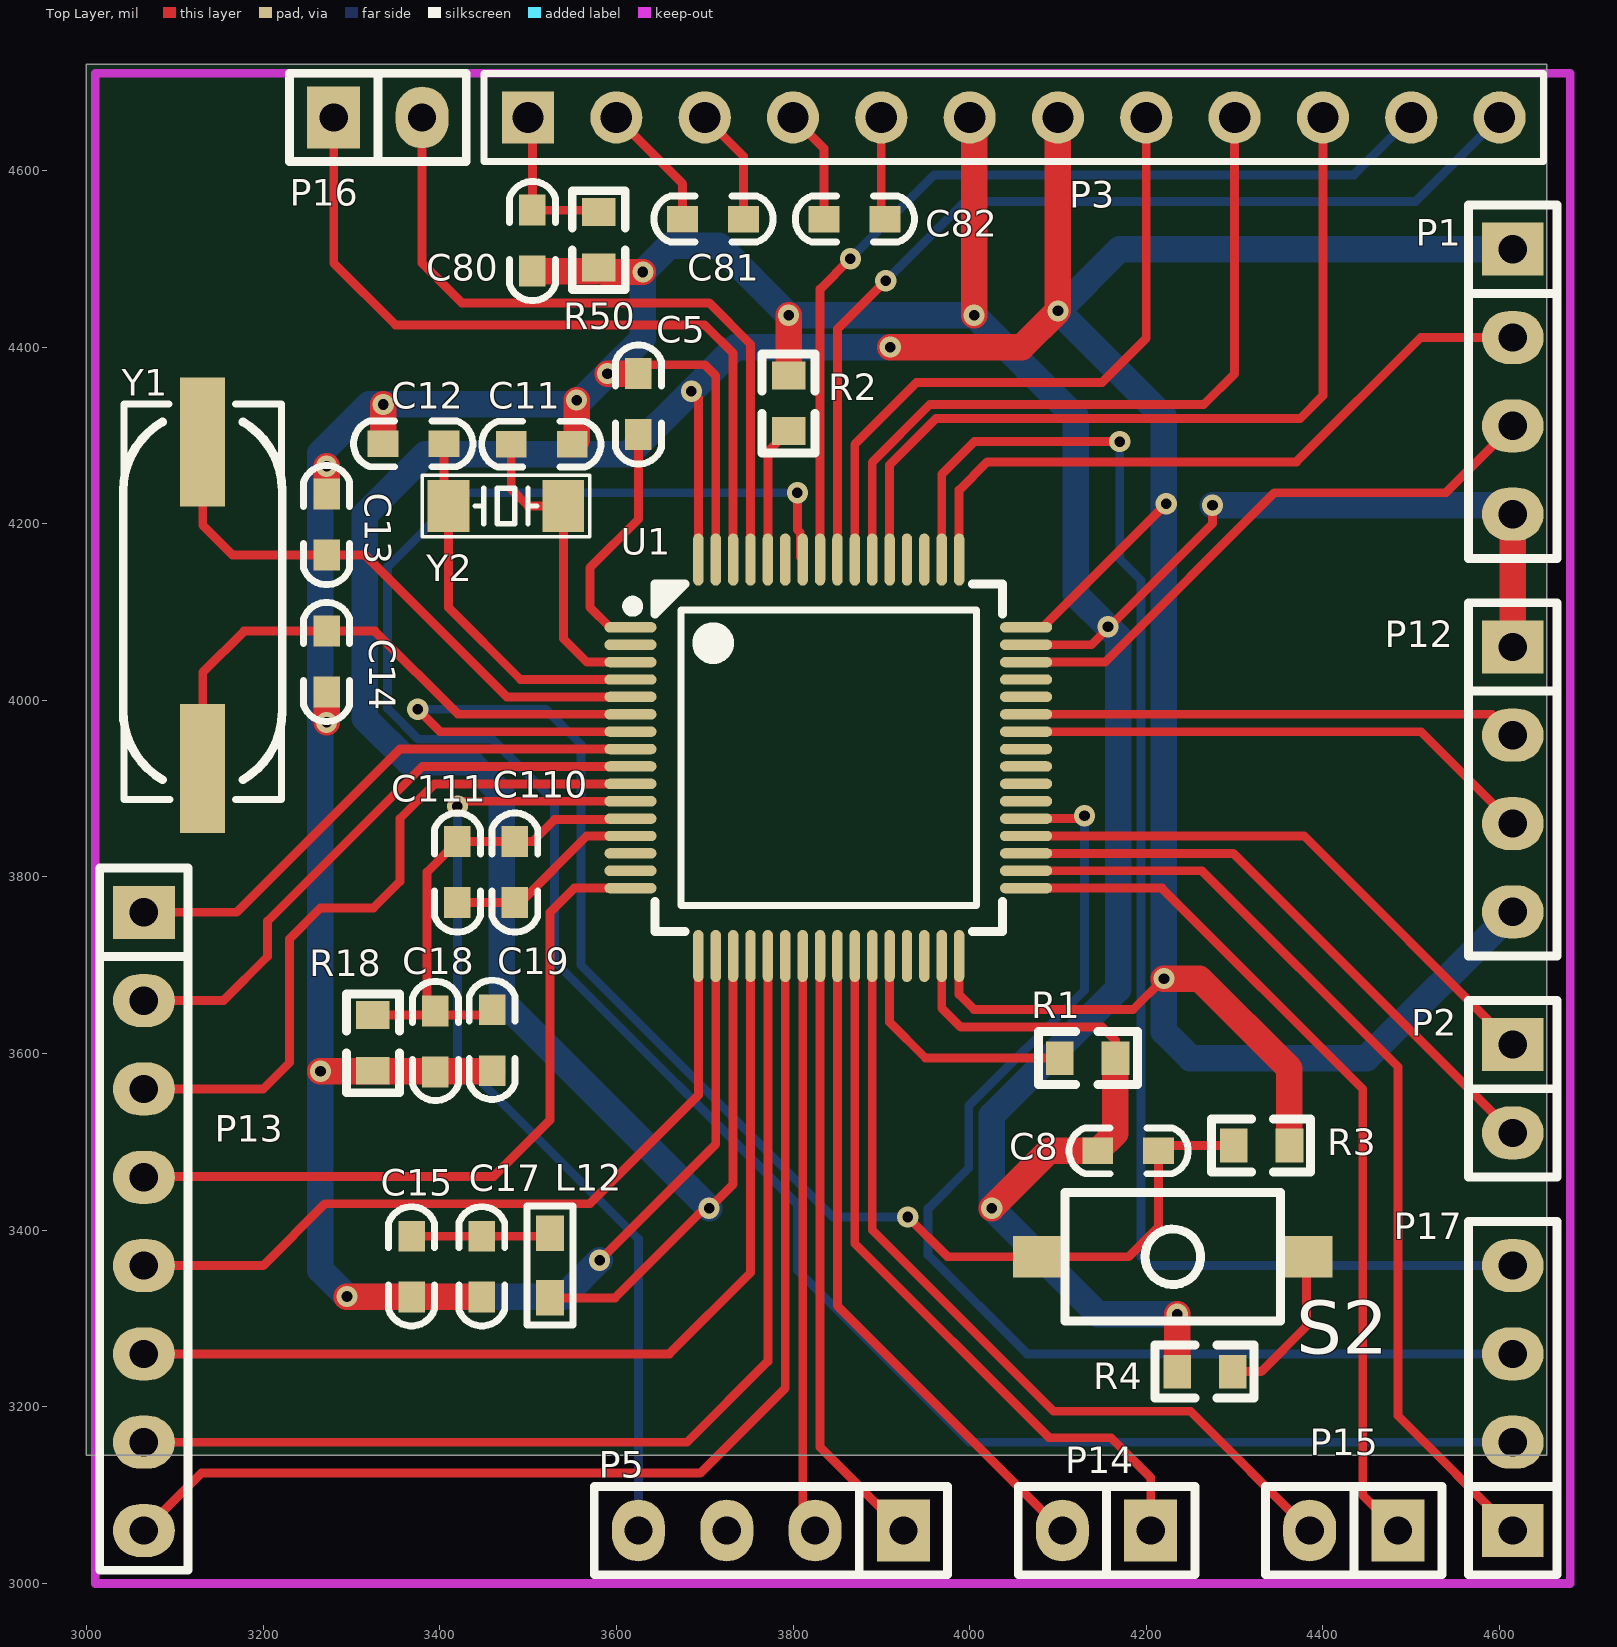
[diagram p0: Top Layer view]
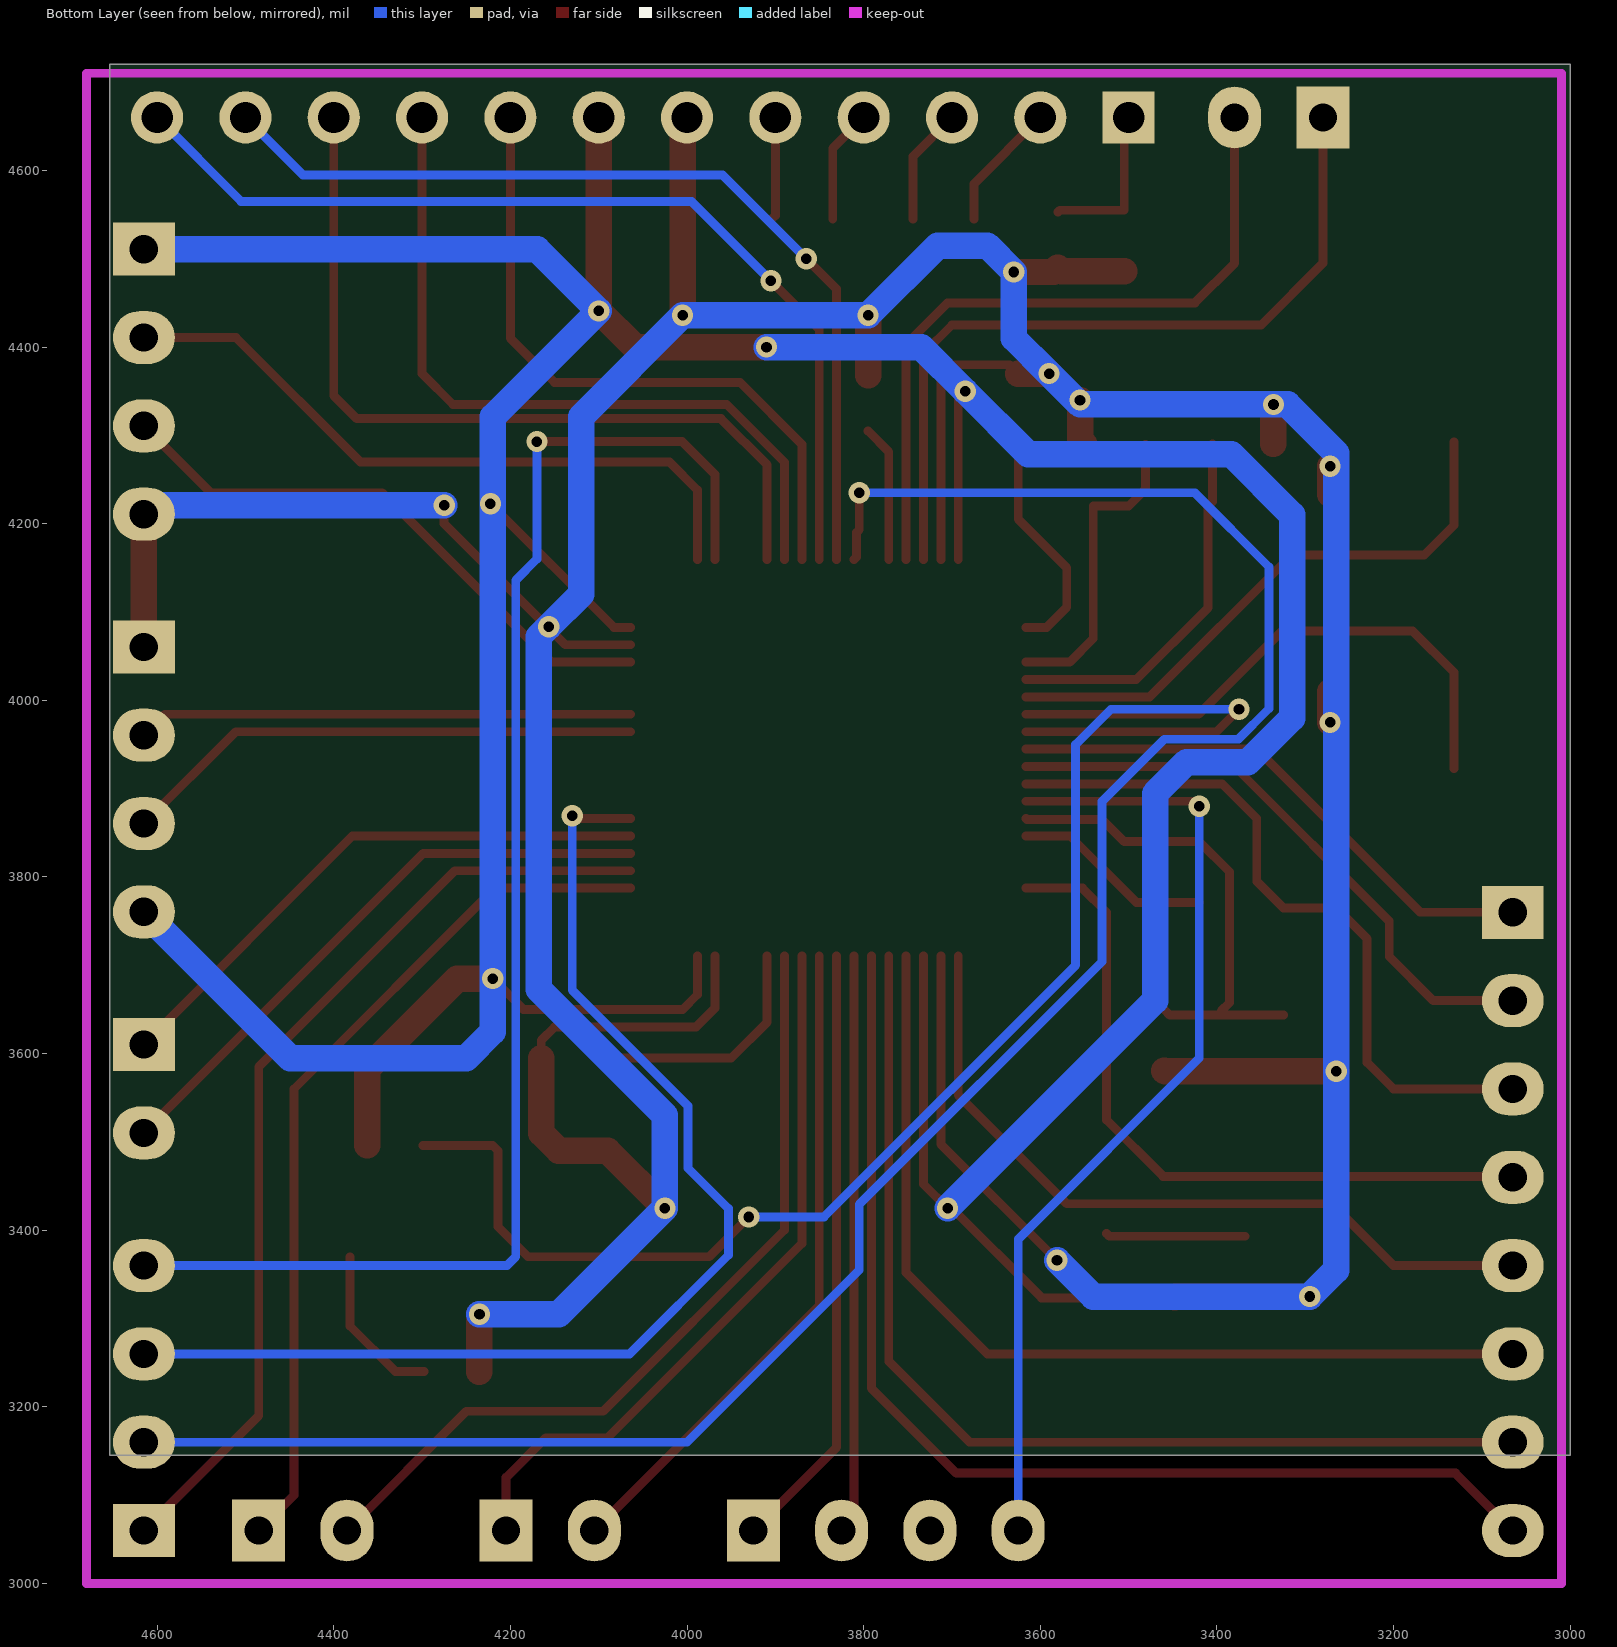
[diagram p1: Bottom Layer view, seen from below]
# Altium PCB MISC51920.pcbdoc
Units mil, origin at the board's own origin, x right, y up, seen from the top; angles counter-clockwise.
Board outline 1653.54 x 1574.8 mil, 2 copper layers (Top Layer, Bottom Layer); 36 components, 70 nets, 158 pads, 29 vias.

## Layer stack, top to bottom (the 12.6 mil dielectric is the usual default, probably not edited)
Top Solder Mask Layer: solder mask 1.4, FR-4, Dk 4.8
Top Layer: signal copper 1.4
Substrate1: surface 12.6, FR-4, Dk 4.8
Bottom Layer: signal copper 1.4
Bottom Solder Mask Layer: solder mask 1.4, FR-4, Dk 4.8

## Board outline
4653.54,3145.2 3000,3145.2 3000,4720 4653.54,4720

## Design rules (kind name [scope] priority, off if disabled: settings)
BoardOutlineClearance Clearance_1 [All] p2: genericclearance=6 ignorepadtopadclearanceinfootprint=FALSE except(0: Arc-SplitContinuation Track-SplitContinuation SMDPad-SplitContinuation THPad-SplitContinuation Via-SplitContinuation Fill-SplitContinuation Region-SplitContinuation Poly-SplitContinuation Text-SplitContinuation Hole-SplitContinuation; 6: Arc-OutlineEdge Track-OutlineEdge SMDPad-OutlineEdge THPad-OutlineEdge Via-OutlineEdge Fill-OutlineEdge Region-OutlineEdge Poly-OutlineEdge Text-OutlineEdge Hole-OutlineEdge SMDPad-CutoutEdge THPad-CutoutEdge Via-CutoutEdge Fill-CutoutEdge Region-CutoutEdge Poly-CutoutEdge Text-CutoutEdge; 6.9: Hole-CutoutEdge; 11.8: Arc-CutoutEdge Track-CutoutEdge)
Clearance [All] p1: gap=6 ignorepadtopadclearanceinfootprint=FALSE
Creepage creepage [All] p1: checkdistance=0 ignoreinternallayers=TRUE applytopolygonpour=TRUE
DiffPairsRouting [All] p1: maxlimit=10 minlimit=6 mostfreqgap=6 toplayer_minwidth=0 toplayer_prefwidth=0 toplayer_maxwidth=0 toplayer_mingap=10 toplayer_prefgap=10 toplayer_maxgap=10 bottomlayer_minwidth=0 bottomlayer_prefwidth=0 bottomlayer_maxwidth=0 bottomlayer_mingap=10 bottomlayer_prefgap=10 bottomlayer_maxgap=10 maxuncoupledlength=10
HoleToHoleClearance ComponentClearance [All] p1: gap=11.81 allowstackedmicrovias=TRUE
Length netLength [All] p1: minlimit=0 maxlimit=0
MatchedLengths netLengthTolerance [All] p1: tolerance=1000
PolygonConnect [(InNet('TIM3_CH1') OR InNet('ADC_IN14'))] p1: connectstyle=Relief reliefconductorwidth=10 reliefentries=4 polygonreliefangle="90 Angle" airgapwidth=10 via.connectstyle=Relief via.reliefconductorwidth=10 via.reliefentries=4 via.polygonreliefangle="90 Angle" via.airgapwidth=10
RoutingVias [All] p1: holewidth=15 width=30 viastyle="Through Hole" minholewidth=12 minwidth=22 maxholewidth=15 maxwidth=30
SolderMaskExpansion [All] p1: expansion=4 istentingtop=FALSE
Width [All] p1: maxlimit=10 minlimit=10 preferedwidth=10 toplayer_minwidth=8 toplayer_maxwidth=30 toplayer_prefwidth=10 bottomlayer_minwidth=8 bottomlayer_maxwidth=30 bottomlayer_prefwidth=10
2 further rules are at their usual default settings.

## Components (designator, comment, footprint, x,y, rotation, side; value= is the part's Value field where it differs from the comment)
C5 "1uF" "C 0603" 3625,4335 r270 top
C8 "104" "C 0603" 4180,3490 r0 top
C11 "20P" "C 0603" 3515,4290 r180 top
C12 "20P" "C 0603" 3370,4290.51 r180 top
C13 "20P" "C 0603" 3271.92,4198.46 r270 top
C14 "20P" "C 0603" 3271.92,4043.46 r270 top
C15 "1uF" "C 0603" 3368.05,3359.22 r90 top
C17 "0.01uF" "C 0603" 3447.61,3359.22 r90 top
C18 "1uF" "C 0603" 3395.19,3614.41 r90 top
C19 "0.01uF" "C 0603" 3459.41,3615.66 r90 top
C80 "330pF" "C 0603" 3505,4520 r270 top
C81 "2.2uF" "C 0603" 3710,4545 r0 top
C82 "2.2uF" "C 0603" 3870,4545 r0 top
C110 "0.1uF" "C 0603" 3485,3805 r270 top
C111 "0.01uF" "C 0603" 3420,3805 r270 top
L12 "2uH" "R 0603" 3525,3360 r270 top
P1 "Pin HDR1X4" "Pin HDR1X4/2.54mm-S" 4615,4510.8 r0 top
P2 "Pin HDR1X2" "Pin HDR1X2/2.54mm-S" 4615,3610.27 r0 top
P3 "Pin HDR1X12" "Pin HDR1X12/2.54mm-S" 3500,4660 r0 top
P5 "Pin HDR1X4" "Pin HDR1X4/2.54mm-S" 3925,3060 r270 top
P12 "Pin HDR1X4" "Pin HDR1X4/2.54mm-S" 4615,4060.53 r0 top
P13 "Pin HDR1X8" "Pin HDR1X8/2.54mm-S" 3065,3760 r0 top
P14 "Pin HDR1X2" "Pin HDR1X2/2.54mm-S" 4205,3060 r270 top
P15 "Pin HDR1X2" "Pin HDR1X2/2.54mm-S" 4485,3060 r270 top
P16 "Pin HDR1X2" "Pin HDR1X2/2.54mm-S" 3280,4660 r90 top
P17 "Pin HDR1X4" "Pin HDR1X4/2.54mm-S" 4615,3060 r180 top
R1 "10K" 0603R 4165,3595 r180 top
R2 "10K" 0603R 3795,4305 r90 top
R3 "10K" 0603R 4299,3496 r0 top
R4 "330R" 0603R 4235,3240 r0 top
R18 "0R" 0603R 3324.41,3580.66 r90 top
R50 "3.3-10M" 0603R 3580,4490 r90 top
S2 "KEY" SWTP3.7X6 4230,3370 r180 top
U1 "STM32L152RBT6" LQFP-64_L10.0-W10.0-P0.50-LS12.0-BL 3840,3935 r270 top
Y1 "8MHz" XTAL_SMD49S 3131.6,3922.69 r270 top
Y2 "32.768kHz" "OSC 3215-2P" 3475,4220 r180 top

## Footprints (in the part's own frame and the unit in brackets; to place one, negate y for a bottom-side part, rotate by r counter-clockwise, add the part's x,y. Pads: shape width x height; smd on the part's side, far side on the other; paste and mask are expansions set on the pad)
0603R [mm]
  rect 0.8x0.965 smd: 1(0,0) 2(1.6,0)
  silkscreen extent -0.64,-0.76 2.21,0.76
"C 0603" [mil]
  rect 35x30 smd: 1(-35,0) 2(34,0)
  silkscreen extent -67,-26 67,26
LQFP-64_L10.0-W10.0-P0.50-LS12.0-BL [mm]
  oval 0.3x1.5 smd: 1(-3.75,-5.688) 2(-3.25,-5.688) 3(-2.75,-5.688) 4(-2.25,-5.688) 5(-1.75,-5.688) 6(-1.25,-5.688) 7(-0.75,-5.688) 8(-0.25,-5.688) 9(0.25,-5.688) 10(0.75,-5.688) 11(1.25,-5.688) 12(1.75,-5.688) 13(2.25,-5.688) 14(2.75,-5.688) 15(3.25,-5.688) 16(3.75,-5.688) 33(3.75,5.688) 34(3.25,5.688) 35(2.75,5.688) 36(2.25,5.688) 37(1.75,5.688) 38(1.25,5.688) 39(0.75,5.688) 40(0.25,5.688) 41(-0.25,5.688) 42(-0.75,5.688) 43(-1.25,5.688) 44(-1.75,5.688) 45(-2.25,5.688) 46(-2.75,5.688) 47(-3.25,5.688) 48(-3.75,5.688)
  oval 1.5x0.3 smd: 17(5.7,-3.738) 18(5.7,-3.238) 19(5.7,-2.738) 20(5.7,-2.238) 21(5.7,-1.738) 22(5.7,-1.238) 23(5.7,-0.738) 24(5.7,-0.238) 25(5.7,0.262) 26(5.7,0.762) 27(5.7,1.262) 28(5.7,1.762) 29(5.7,2.262) 30(5.7,2.762) 31(5.7,3.262) 32(5.7,3.762) 49(-5.7,3.762) 50(-5.7,3.262) 51(-5.7,2.762) 52(-5.7,2.262) 53(-5.7,1.762) 54(-5.7,1.262) 55(-5.7,0.762) 56(-5.7,0.262) 57(-5.7,-0.238) 58(-5.7,-0.738) 59(-5.7,-1.238) 60(-5.7,-1.738) 61(-5.7,-2.238) 62(-5.7,-2.738) 63(-5.7,-3.238) 64(-5.7,-3.738)
  silkscreen extent -5,-5.78 5,5.01
"OSC 3215-2P" [mm]
  rect 1.2x1.5 smd: 1(-1.65,0) 2(1.65,0)
  silkscreen extent -2.41,-0.89 2.41,0.89
"Pin HDR1X2/2.54mm-S" [mil]
  rect 70x60 hole 32: 1(0,0)
  oval 70x60 hole 32: 2(0,-100)
  silkscreen extent -50,-150 50,50
"Pin HDR1X4/2.54mm-S" [mil]
  rect 70x60 hole 32: 1(0,0)
  oval 70x60 hole 32: 2(0,-100) 3(0,-200) 4(0,-300)
  silkscreen extent -50,-350 50,50
"Pin HDR1X8/2.54mm-S" [mil]
  rect 70x60 hole 32: 1(0,0)
  oval 70x60 hole 32: 2(0,-100) 3(0,-200) 4(0,-300) 5(0,-400) 6(0,-500) 7(0,-600) 8(0,-700)
  silkscreen extent -50,-745 50,50
"Pin HDR1X12/2.54mm-S" [mm]
  rect 1.5x1.5 hole 0.9: 1(0,0)
  round 1.5 hole 0.9: 2(2.54,0) 3(5.08,0) 4(7.62,0) 5(10.16,0) 6(12.7,0) 7(15.24,0) 8(17.78,0) 9(20.32,0) 10(22.86,0) 11(25.4,0) 12(27.94,0)
  silkscreen extent -1.27,-1.27 29.21,1.27
"R 0603" [mil]
  rect 40x31.5 smd: 1(-36.5,0) 2(36.5,0)
  silkscreen extent -68,-26 68,26
SWTP3.7X6 [mm]
  rect 1.5x1.2 smd: 1(-3.85,0) 2(3.85,0)
  silkscreen extent -3.1,-1.85 3.1,1.85
XTAL_SMD49S [mil]
  rect 146x51 smd: 1(0,0) 2(-370,0)
  silkscreen extent -413,-90 35,90

## Via types
v1: diameter 24.02, hole 12, Top Layer to Bottom Layer, 29 vias

## Nets (pads, with @x,y where several pads share a name; then routed paths per layer and width w, separated by ;. In a path a pad name is that pad's centre, name@x,y a point inside that pad or via, vN(x,y) a via of type N, cw(c..) or ccw(c..) an arc to the next point about the centre after c; other vN are vias at no path point)
+3.3V: L12.2 P1.1 P3.7 P12.4 R3.2 U1.19 U1.32 U1.48 U1.64 | length 5468.9
  Top Layer w10: L12.2 3598.5,3323.5 v1@3702.5,3427.5 ; v1(3685,4350) 3692.83,4342.17 U1.64 ; v1(3705,3425) 3732.2,3452.2 U1.19 ; U1.32 3988.11,3666.89 4005,3650 4185,3650 v1(4220,3685) ; U1.48 4082.64,4082.64 v1(4222.64,4222.64)
  Top Layer w30: v1(3910,4400) 4059,4400 v1(4100,4441) P3.7 ; v1(4220,3685) 4260,3685 4361.99,3583.01 R3.2
  Bottom Layer w30: v1(3705,3425) 3470,3660 3470,3894.46 3434.46,3930 3365,3930 3315,3980 3315,4210 3383.86,4278.86 3613.86,4278.86 v1(3685,4350) 3735,4400 v1(3910,4400) ; P12.4 4449.47,3595 4249.89,3595 4220,3624.89 v1(4220,3685) 4220,4321 v1(4100,4441) 4169.8,4510.8 P1.1
ADC_IN1: U1.15
ADC_IN2: P13.4 U1.16 | length 824.3
  Top Layer w10: P13.4 3065.95,3460.95 3460.95,3460.95 3525,3525 3525,3760 3552.36,3787.36 U1.16
ADC_IN3: P13.5 U1.17 | length 865.5
  Top Layer w10: P13.5 3200,3360 3270,3430 3570,3430 3692.83,3552.83 U1.17
ADC_IN4: P13.6 U1.20 | length 1083.7
  Top Layer w10: P13.6 3660,3260 3751.89,3351.89 U1.20
ADC_IN5: P13.7 U1.21 | length 1203.5
  Top Layer w10: P13.7 3680,3160 3771.57,3251.57 U1.21
ADC_IN6: P13.8 U1.22 | length 1282.4
  Top Layer w10: P13.8 3130,3125 3695,3125 3791.26,3221.26 U1.22
ADC_IN7: P5.2 U1.23 | length 656.4
  Top Layer w10: U1.23 3810.94,3074.06 P5.2
ADC_IN8: P14.1 U1.26 | length 830.4
  Top Layer w10: U1.26 3870,3385 4090,3165 4160,3165 4205,3120 P14.1
ADC_IN9: P15.2 U1.27 | length 946.6
  Top Layer w10: U1.27 3889.68,3400.32 4095,3195 4250,3195 P15.2
ADC_IN10: P13.1 U1.8 | length 627.6
  Top Layer w10: P13.1 3170,3760 3354.84,3944.84 U1.8
ADC_IN11: P13.2 U1.9 | length 684.3
  Top Layer w10: P13.2 3155,3660 3205,3710 3205,3750 3380.16,3925.16 U1.9
ADC_IN12: P13.3 U1.10 | length 817.9
  Top Layer w10: P13.3 3200,3560 3230,3590 3230,3730 3265,3765 3325,3765 3355,3795 3355,3866.21 3394.26,3905.47 U1.10
ADC_IN13: P5.4 U1.11 | length 1103.4
  Top Layer w10: v1(3420,3880) 3425.79,3885.79 U1.11
  Bottom Layer w10: v1(3420,3880) 3420,3595 3625,3390 P5.4
ADC_IN14: P5.1 U1.24 | length 689.7
  Top Layer w10: U1.24 3830.63,3154.37 P5.1
ADC_IN15: P14.2 U1.25 | length 756.1
  Top Layer w10: U1.25 3850.31,3314.69 P14.2
ADC_IN18: P15.1 U1.33 | length 991.8
  Top Layer w10: U1.33 4217.64,3787.36 4445,3560 4445,3100 P15.1
ADC_IN19: P5.3
ADC_IN20: P2.2 U1.35 | length 682.1
  Top Layer w10: U1.35 4298.54,3826.73 P2.2
ADC_IN21: P2.1 U1.36 | length 648.9
  Top Layer w10: U1.36 4378.85,3846.42 P2.1
LCD_CD: P3.10 U1.53 | length 945.4
  Top Layer w10: U1.53 3909.37,4266.74 3961.63,4319 4374,4319 4400,4345 P3.10
LCD_CS: P3.12 U1.56 | length 1109.9
  Top Layer w10: U1.56 3850.31,4420.31 v1(3905,4475)
  Bottom Layer w10: v1(3905,4475) 3995,4565 4505,4565 P3.12
LCD_D6: P3.9 U1.54 | length 852.1
  Top Layer w10: U1.54 3889.68,4269.68 3955,4335 4265,4335 4300,4370 P3.9
LCD_D7: P3.8 U1.55 | length 760.3
  Top Layer w10: U1.55 3870,4290 3940,4360 4150,4360 4200,4410 P3.8
LCD_RST: P3.11 U1.57 | length 1056.1
  Top Layer w10: U1.57 3830.63,4465.63 v1(3865,4500)
  Bottom Layer w10: v1(3865,4500) 3960,4595 4435,4595 P3.11
NetC5_2: C5.2 U1.1 | length 119.2
  Top Layer w10: U1.1@3592.82,4082.64 U1.1 ; 3625,4205 C5.2
NETC5_2:  | length 154.6
  Top Layer w10: 3592.82,4082.64 3570,4105.46 3570,4150 3625,4205
NetC80_1: C80.1 P3.1 R50.2 | length 107.1
  Top Layer w10: P3.1 3505,4655 C80.1
NETC80_1:  | length 75.8
  Top Layer w10: 3505,4555 3577.99,4555 3580,4552.99
NetC81_1: C81.1 P3.2
NETC81_1:  | length 146.1
  Top Layer w10: 3600,4660 3675,4585 3675,4545
NetC81_2: C81.2 P3.3 | length 62.2
  Top Layer w10: P3.3 3744,4616
NETC81_2:  | length 71
  Top Layer w10: 3744,4545 3744,4616
NetC82_1: C82.1 P3.4 | length 49.5
  Top Layer w10: P3.4 3835,4625
NETC82_1:  | length 80
  Top Layer w10: 3835,4545 3835,4625
NetC82_2: C82.2 P3.5 | length 116.7
  Top Layer w10: P3.5 3900,4549 C82.2
NetR1_2: R1.2 U1.28 | length 75
  Top Layer w10: 3909.37,3635.63 U1.28
NETR1_2:  | length 209.5
  Top Layer w10: 3909.37,3635.63 3950,3595 4102.01,3595
NetR2_1: R2.1 U1.60
NETR2_1:  | length 155.3
  Top Layer w10: 3771.57,4159.41 3771.57,4281.57 3795,4305
NetR4_2: R4.2 S2.1 | length 78.4
  Top Layer w10: 4381.57,3291.57 S2.1
NETR4_2:  | length 104.9
  Top Layer w10: 4297.99,3240 4330,3240 4381.57,3291.57
NetU1_2: U1.2
NetU1_14: U1.14
NetU1_29: U1.29
NetU1_30: U1.30
NRST: C8.2 R3.1 S2.2 U1.7 | length 1681.4
  Top Layer w10: v1(3375,3990) 3400.47,3964.53 U1.7 ; v1(3930,3415) 3975,3370 S2.2 4180,3370 4214,3404 C8.2 4220,3496 R3.1
  Bottom Layer w10: v1(3375,3990) 3520,3990 3560,3950 3560,3700 3845,3415 v1(3930,3415)
OSC_8M_IN: C13.2 U1.5 Y1.2 | length 659.3
  Top Layer w10: Y1.2 3131.6,4198.4 3165.54,4164.46 C13.2 3315.54,4164.46 3476.1,4003.9 U1.5
OSC_8M_OUT: C14.1 U1.6 Y1.1 | length 651.8
  Top Layer w10: Y1.1 3131.6,4031.6 3178.46,4078.46 C14.1 3326.54,4078.46 3420.79,3984.21 U1.6
OSC_32_IN: C11.2 U1.3 Y2.1 | length 355
  Top Layer w10: C11.2 3481,4239 3500,4220 Y2.1 3539.96,4070.04 3566.73,4043.27 U1.3
OSC_32_OUT: C12.1 U1.4 Y2.2 | length 427.4
  Top Layer w10: C12.1 3405,4225.04 Y2.2 3410.04,4104.96 3491.42,4023.58 U1.4
PA12: U1.45
RST: U1.41
SLEEP: U1.44
SWCLK: P1.2 U1.49 | length 777.1
  Top Layer w10: U1.49 3988.11,4238.11 4020,4270 4370,4270 4510.8,4410.8 P1.2
SWDIO: P1.3 U1.46 | length 661.9
  Top Layer w10: U1.46 4153.27,4043.27 4345,4235 4539.2,4235 P1.3
TIM2_CH1: P17.4 U1.50 | length 1671.6
  Top Layer w10: U1.50 3968.42,4256.04 4005.38,4293.01 v1(4170,4293.01)
  Bottom Layer w10: v1(4170,4293.01) 4170,4160 4194,4136 4194,3370 4204,3360 P17.4
TIM3_CH1: P17.3 U1.37 | length 1346.6
  Top Layer w10: U1.37 4126.67,3866.1 v1(4130,3869.43)
  Bottom Layer w10: v1(4130,3869.43) 4130,3671.77 3999,3540.77 3999,3470.52 3953.01,3424.53 3953.01,3371.99 4065,3260 P17.3
TIM4_CH1: P17.2 U1.58 | length 2504.9
  Top Layer w10: v1(3805,4235) 3805,4193.2 3808.16,4190.03 3808.16,4162.18 U1.58
  Bottom Layer w10: v1(3805,4235) 3425,4235 3341,4151 3341,3990.77 3375.77,3956 3459.59,3956 3530,3885.59 3530,3704.26 3805,3429.26 3805,3355 4000,3160 P17.2
TIM9_CH1: P17.1 U1.34 | length 1091.9
  Top Layer w10: U1.34 4262.95,3807.05 4485,3585 4485,3190 P17.1
TIM10_CH1: P16.2 U1.61 | length 818.7
  Top Layer w10: P16.2 3380,4495 3425,4450 3705,4450 3751.89,4403.11 U1.61
TIM11_CH1: P16.1 U1.62 | length 892.9
  Top Layer w10: P16.1 3280,4495 3350,4425 3700,4425 3732.2,4392.8 U1.62
USART1_RX: P12.2 U1.43 | length 560.9
  Top Layer w10: U1.43 4591.32,3984.21 P12.2
USART1_TX: P12.3 U1.42 | length 594.1
  Top Layer w10: U1.42 4511,3964.53 P12.3
USART3_RX: U1.52
USART3_TX: U1.51
VCC_A: C110.2 C111.2 U1.13 | length 227.3
  Top Layer w10: C111.2 C110.2 3491,3771 3566.42,3846.42 U1.13
VCCA: C15.2 C17.2 L12.1 | length 158.3
  Top Layer w10: C15.2 C17.2 3521.72,3393.22 L12.1
VSS_1: C5.1 C8.1 C11.1 C12.2 C13.1 C14.2 C15.1 C17.1 C18.1 C19.1 C80.2 P1.4 P3.6 P12.1 R1.1 R2.2 R4.1 R18.1 R50.1 U1.18 U1.31 U1.47 U1.63 | length 6652.8
  Top Layer w10: v1(3581.05,3366.05) 3712.52,3497.52 U1.18 ; C5.1 3635,4380 3700,4380 3712.52,4367.48 U1.63 ; U1.31 3968.42,3651.58 3990,3630 4150,3630 4165,3615 R1.1 ; U1.47 4137.95,4062.95 4275,4200 v1(4275,4220.8)
  Top Layer w30: v1(3265,3580) 3458.75,3580 C19.1 ; v1(3271.92,3975) C14.2 ; C13.1 v1(3271.92,4265) ; v1(3295,3325) 3446.83,3325 C17.1 ; C12.2 v1(3336,4335) ; C80.2 3576,4486 R50.1 3585,4485 v1(3630,4485) ; C11.1 3555,4295 v1(3555,4340) ; v1(3590,4370) C5.1 ; R2.2 v1(3795,4436) ; P3.6 4005,4655 v1(4005,4436) ; v1(4025,3425) 4090,3490 C8.1 4165,3510 R1.1 ; R4.1 v1(4235,3305) ; P12.1 P1.4
  Bottom Layer w30: v1(3581.05,3366.05) 3540,3325 v1(3295,3325) 3265,3355 v1(3265,3580) 3265,4280 3320,4335 v1(3336,4335) 3555,4335 v1(3590,4370) 3630,4410 v1(3630,4485) 3660,4515 3716,4515 v1(3795,4436) v1(4005,4436) 4120,4321 4120,4120 v1(4156.65,4083.35) 4168,4072 4168,3673 4025,3530 v1(4025,3425) 4145,3305 v1(4235,3305) ; v1(4275,4220.8) 4605,4220.8 P1.4
VSS_A: C18.2 C19.2 C110.1 C111.1 R18.2 U1.12 | length 554.1
  Top Layer w10: R18.2 3453.4,3643.65 C19.2 ; C18.2 3385.71,3657.88 3385.71,3805.71 C111.1 C110.1 3505,3840 3530,3865 3614.96,3865 U1.12
pads on no net: U1.38 U1.39 U1.40 U1.59

## Keep-outs
Board Outline Layer:
  lines w10: 3010,3000 3010,4710 4680,4710 4680,3000 3010,3000